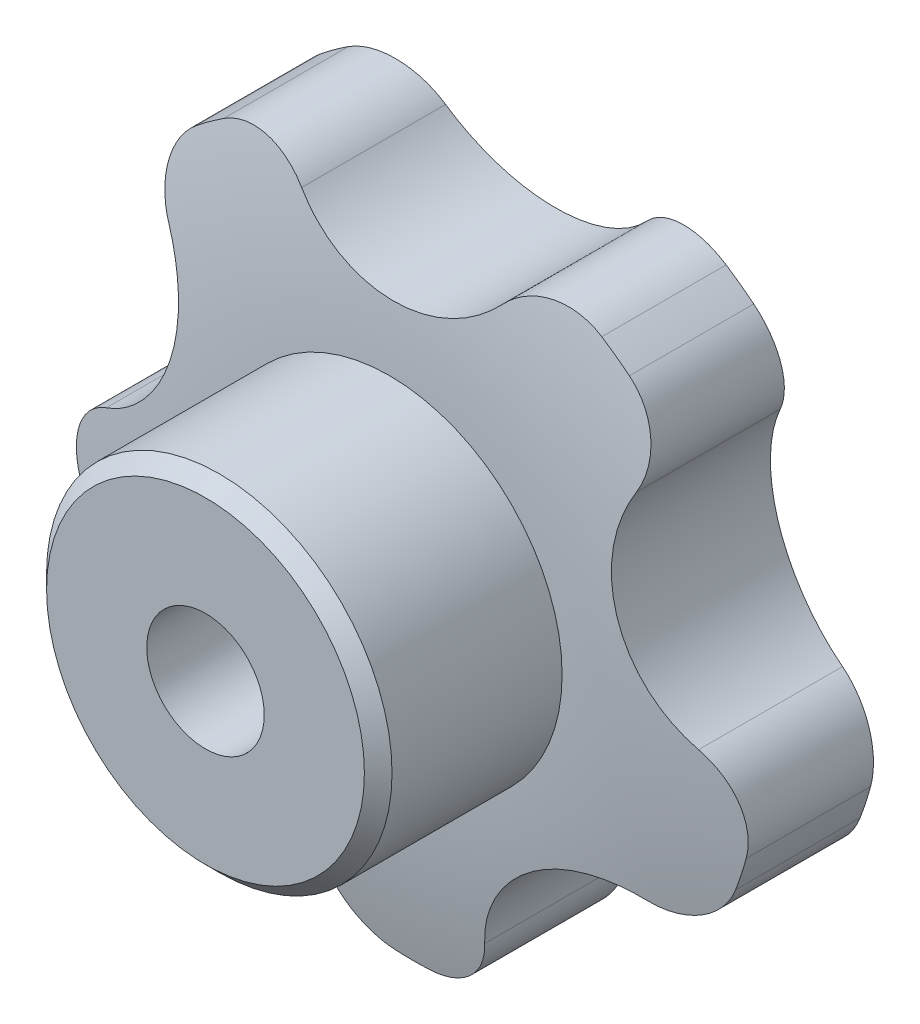
SolidWorks part; units mm, degrees
material "45"
ref_plane "前视基准面" through (0, 0, 0) normal (0, 0, 1) x (1, 0, 0)
ref_plane "上视基准面" through (0, 0, 0) normal (0, 1, 0) x (1, 0, 0)
ref_plane "右视基准面" through (0, 0, 0) normal (1, 0, 0) x (0, 0, -1)
sketch "草图1" plane through (0, 0, 0) normal (0, 1, 0) x (1, 0, 0)
  line L0 (0, 58.4884) -> (0, -35.4651) construction
  line L2 (25, 24) -> (25, 15)
  line L4 (12.5, 13.308) -> (12.5, 0)
  line L5 (12.5, 0) -> (0, 0)
  line L6 (0, 0) -> (0, 26)
  arc A0 (0, 26) -> (25, 24) centre (4.5081, -74.8993) cw
  arc A1 (25, 15) -> (12.5, 13.308) centre (10.3865, 75.943) cw
  dimension "D6" = 101
  dimension "D8" = 62.6706
  dimension "D1" = 26
  dimension "D2" = 12.5
  dimension "D3" = 24
  dimension "D4" = 15
  dimension "D5" = 25
  dimension "D7" = 13.308
revolve "旋转1" add sketch "草图1" angle 360 about L0
hole_wizard "M10 螺纹孔1" positions "草图3" profile "草图2" tap size "M10" standard "ISO"
sketch "草图3" plane through (0, 0, 0) normal (0, 0, 1) x (1, 0, 0)
  point P0 (0, 0)
sketch "草图2" plane through (0, 0, 0) normal (1, 0, 0) x (0, -1, 0)
  line L0 (0, 0) -> (0, 22.0537)
  line L1 (0, 22.0537) -> (4.25, 19.5)
  line L2 (4.25, 19.5) -> (4.25, 0)
  line L5 (4.25, 0) -> (0, 0)
  line L10 (0, 22.0537) -> (-4.25, 19.5) construction
  line L11 (0, -6.35) -> (0, 107.95) construction
  dimension "螺纹孔钻头直径" = 8.5
  dimension "螺纹孔钻头深度" = 19.5
  dimension "导头角度" = 118
cosmetic thread "孔螺蚊线1" parameters "D1"=15, "D2"=10
sketch "草图4" plane through (0, 0, 0) normal (0, 0, 1) x (1, 0, 0)
  line L0 (0, 27.3437) -> (0, -22.855) construction
  line L1 (-24.239, 0) -> (27.1567, 0) construction
  circle A0 centre (0, 27) radius 10
  dimension "D1" = 20
  dimension "D2" = 27
extrude "切除-拉伸2" cut sketch "草图4" against normal blind 36
pattern_circular "阵列(圆周)1" count 5 every 72 about axis through (0, 0, 0) along (0, 0, 1) of "切除-拉伸2"
fillet "圆角2" radius 5 10 edges at (-24.9468, -1.6297, -19.5) (-19.2245, 15.9819, -19.5) (-9.259, 23.2222, -19.5) (9.259, 23.2222, -19.5) (-6.159, -24.2295, -19.5) (-21.1403, -13.3449, -19.5) (21.1403, -13.3449, -19.5) (6.159, -24.2295, -19.5) (19.2245, 15.9819, -19.5) (24.9468, -1.6297, -19.5)
chamfer "倒角1" distance 1 angle 45 1 edges at (-12.5, 0, 0)
